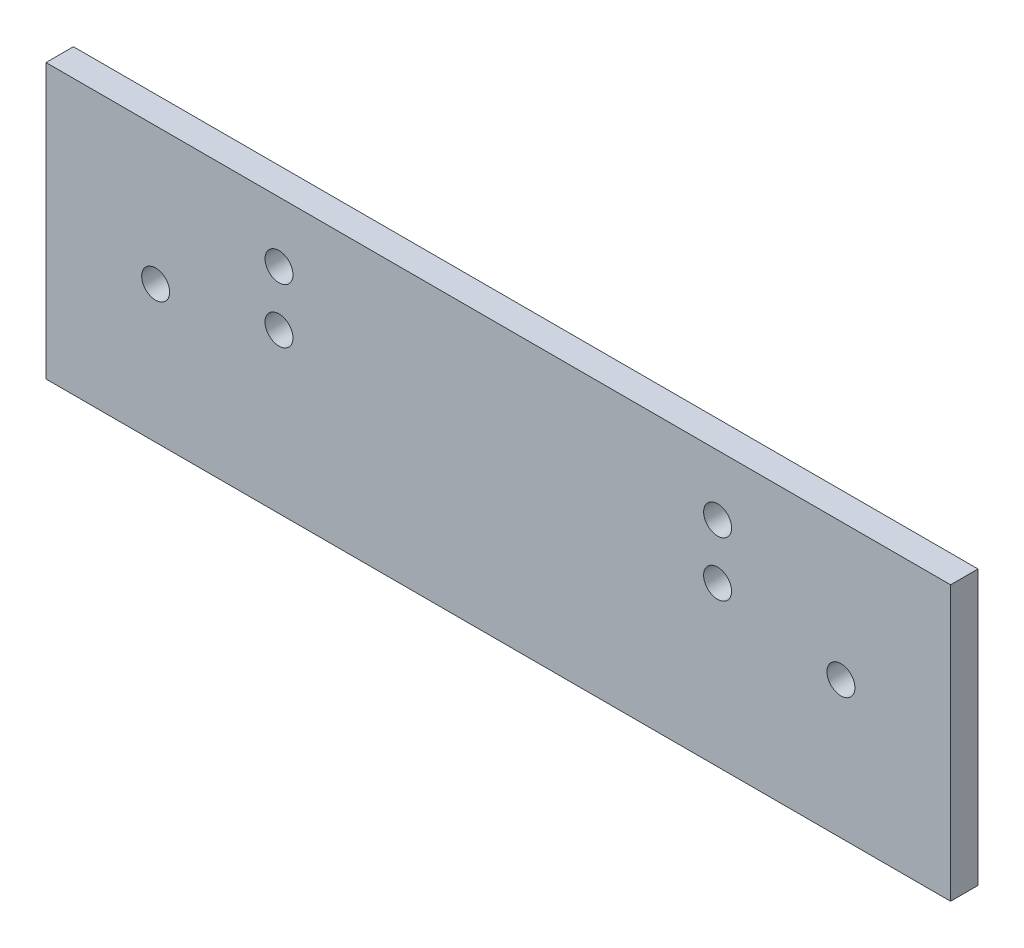
SolidWorks part; units mm, degrees
material "1023 碳钢板 (SS)"
ref_plane "Front Plane" through (0, 0, 0) normal (0, 0, 1) x (1, 0, 0)
ref_plane "Top Plane" through (0, 0, 0) normal (0, 1, 0) x (1, 0, 0)
ref_plane "Right Plane" through (0, 0, 0) normal (1, 0, 0) x (0, 0, -1)
sketch "Sketch1" plane through (0, 0, 0) normal (0, 0, 1) x (1, 0, 0)
  line L1 (-165, 50) -> (165, 50)
  line L2 (-165, 50) -> (-165, -50)
  line L3 (-165, -50) -> (165, -50)
  line L4 (165, 50) -> (165, -50)
  line L5 (-165, 50) -> (165, -50) construction
  line L6 (-165, -50) -> (165, 50) construction
  point P0 (0, 0)
  dimension "D1" = 330
  dimension "D2" = 100
extrude "Boss-Extrude1" add sketch "Sketch1" along normal blind 10 contours L2 L1 L4 L3
sketch "Sketch2" plane through (0, 0, 10) normal (0, 0, 1) x (1, 0, 0)
  line L0 (-165, -50) -> (165, -50) construction
  circle A0 centre (-80, 28) radius 4.5
  circle A1 centre (80, 28) radius 4.5
  circle A2 centre (-80, 8) radius 4.5
  circle A3 centre (80, 8) radius 4.5
  circle A4 centre (-125, 0) radius 4.5
  circle A5 centre (125, 0) radius 4.5
  dimension "D8" = 9
  dimension "D1" = 160
  dimension "D2" = 80
  dimension "D3" = 20
  dimension "D4" = 58
  dimension "D5" = 50
  dimension "D6" = 125
  dimension "D7" = 250
hole_wizard "M12 Tapped Hole1" positions "Sketch3" profile "Sketch4" tap size "M12" standard "ISO"
sketch "Sketch3" plane through (0, 0, 10) normal (0, 0, 1) x (1, 0, 0)
  point P0 (-125, 0)
  point P3 (-80, 8)
  point P6 (-80, 28)
  point P9 (80, 28)
  point P12 (80, 8)
  point P15 (125, 0)
sketch "Sketch4" plane through (-125, 0, 10) normal (1, 0, 0) x (0, -1, 0)
  line L0 (0, 0) -> (0, 32.3144)
  line L1 (0, 32.3144) -> (5.1, 29.25)
  line L2 (5.1, 29.25) -> (5.1, 0)
  line L5 (5.1, 0) -> (0, 0)
  line L10 (0, 32.3144) -> (-5.1, 29.25) construction
  line L11 (0, -6.35) -> (0, 107.95) construction
  dimension "螺纹孔钻头直径" = 10.2
  dimension "螺纹孔钻头深度" = 29.25
  dimension "导头角度" = 118
cosmetic thread "Hole Thread Line 1"
cosmetic thread "Hole Thread Line 2"
cosmetic thread "Hole Thread Line 3"
cosmetic thread "Hole Thread Line 4"
cosmetic thread "Hole Thread Line 5"
cosmetic thread "Hole Thread Line 6"
